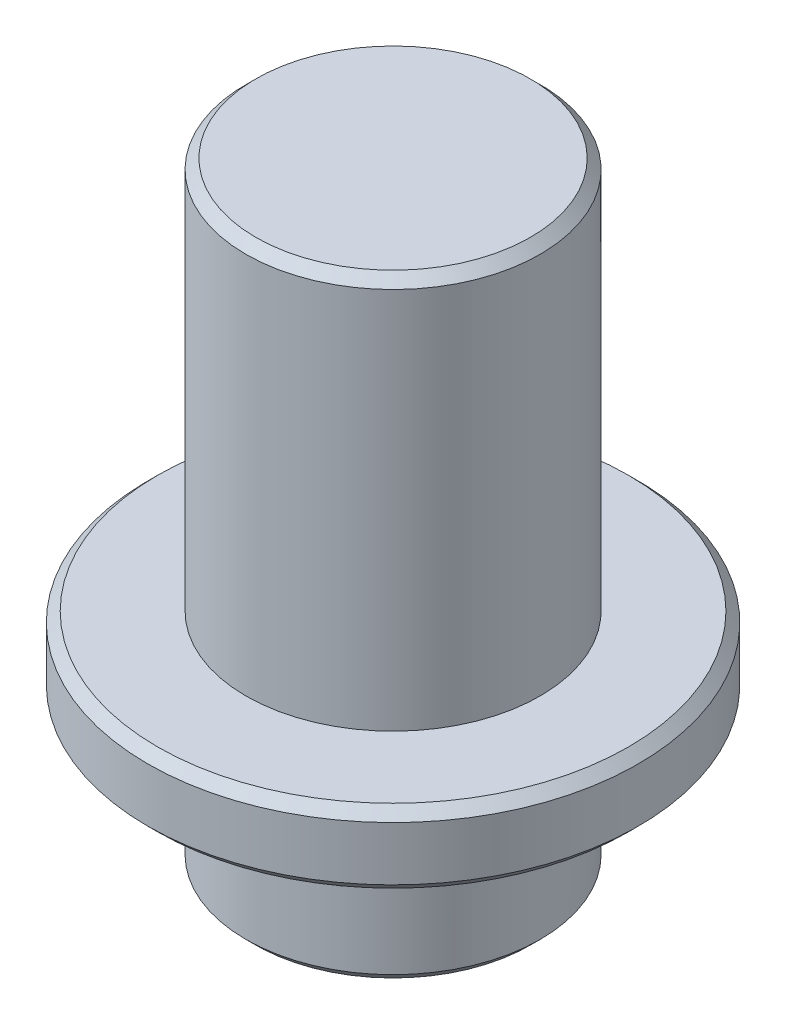
SolidWorks part; units mm, degrees
material "Plain carbon steel"
ref_plane "Front Plane" through (0, 0, 0) normal (0, 0, 1) x (1, 0, 0)
ref_plane "Top Plane" through (0, 0, 0) normal (0, 1, 0) x (1, 0, 0)
ref_plane "Right Plane" through (0, 0, 0) normal (1, 0, 0) x (0, 0, -1)
sketch "Sketch1" plane through (0, 0, 0) normal (0, 1, 0) x (1, 0, 0)
  circle A0 centre (0, 0) radius 5
  dimension "D1" = 10
extrude "Boss-Extrude1" add sketch "Sketch1" along normal blind 1.5
sketch "Sketch2" plane through (0, 1.5, 0) normal (0, 1, 0) x (1, 0, 0)
  circle A0 centre (0, 0) radius 3
  dimension "D1" = 6
extrude "Boss-Extrude2" add sketch "Sketch2" along normal blind 8
sketch "Sketch3" plane through (0, 0, 0) normal (0, -1, 0) x (1, 0, 0)
  circle A0 centre (0, 0) radius 3
  dimension "D1" = 6
extrude "Boss-Extrude3" add sketch "Sketch3" along normal blind 3
chamfer "Chamfer1" distance 0.2 angle 45 4 edges at (0, -3, -3) (0, 0, 5) (0, 1.5, 5) (0, 9.5, 3)
